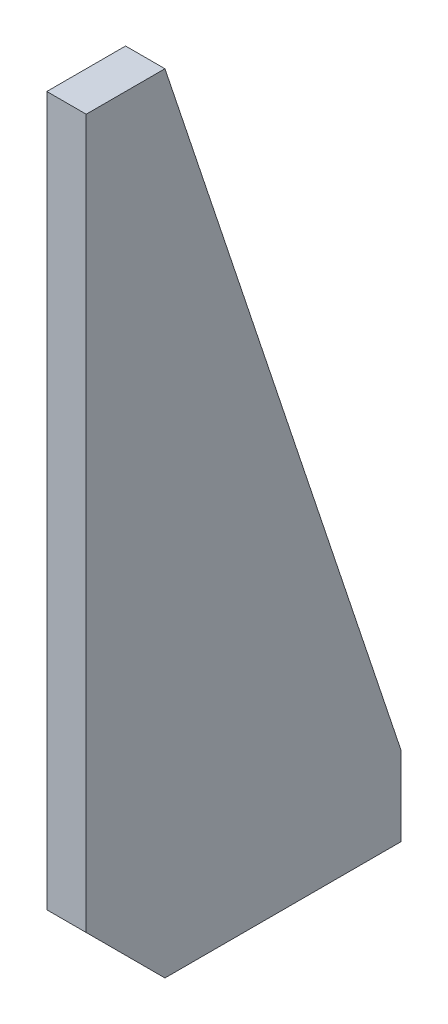
from build123d import *

# Parameters (mm, degrees)
BOSS_EXTRUDE1_DEPTH = 10


with BuildPart() as part:
    # Sketch1 → Boss-Extrude1 (new body)
    with BuildSketch(Plane(origin=(0, 0, 0), x_dir=(0, 0, -1), z_dir=(1, 0, 0))):
        Polygon((40, -80), (-20, 100), (-40, 100), (-40, -80), (-20, -100), (40, -100), align=None)
    extrude(amount=BOSS_EXTRUDE1_DEPTH)


solid = part.part
